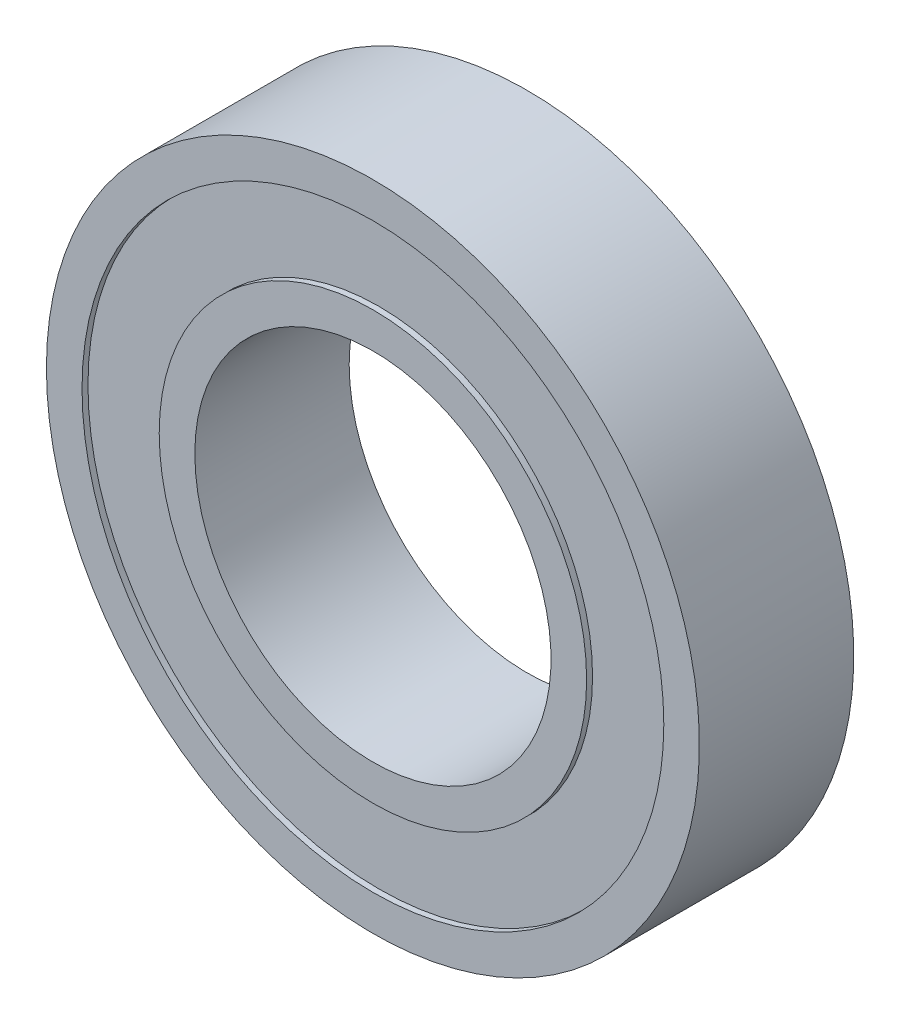
SolidWorks part; units mm, degrees
material "SS41"
ref_plane "Front Plane" through (0, 0, 0) normal (0, 0, 1) x (1, 0, 0)
ref_plane "Top Plane" through (0, 0, 0) normal (0, 1, 0) x (1, 0, 0)
ref_plane "Right Plane" through (0, 0, 0) normal (1, 0, 0) x (0, 0, -1)
sketch "Sketch1" plane through (0, 0, 0) normal (0, 0, 1) x (1, 0, 0)
  circle A0 centre (0, 0) radius 27.5
  circle A1 centre (0, 0) radius 15
  dimension "D1" = 55
  dimension "D2" = 30
extrude "Boss-Extrude1" add sketch "Sketch1" along normal mid plane 13
sketch "Sketch2" plane through (0, 0, 6.5) normal (0, 0, 1) x (1, 0, 0)
  circle A0 centre (0, 0) radius 24.5
  circle A1 centre (0, 0) radius 18
  dimension "D1" = 36
  dimension "D2" = 49
extrude "Cut-Extrude1" cut sketch "Sketch2" against normal blind 0.5
mirror "Mirror1" about plane through (0, 0, 0) normal (0, 0, 1) of "Cut-Extrude1"
